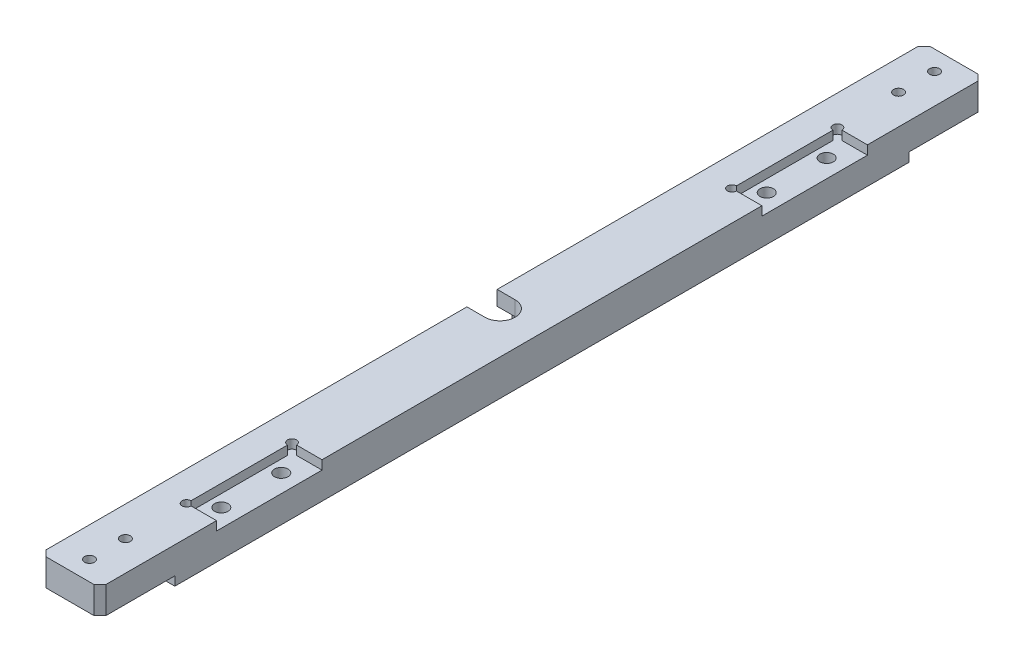
SolidWorks part; units mm, degrees
material "AL6061"
ref_plane "Front Plane" through (0, 0, 0) normal (0, 0, 1) x (1, 0, 0)
ref_plane "Top Plane" through (0, 0, 0) normal (0, 1, 0) x (1, 0, 0)
ref_plane "Right Plane" through (0, 0, 0) normal (1, 0, 0) x (0, 0, -1)
sketch "Sketch1" plane through (0, 0, 0) normal (1, 0, 0) x (0, 0, -1)
  line L1 (-147.5, -6) -> (147.5, -6)
  line L2 (-147.5, -6) -> (-147.5, 6)
  line L3 (-147.5, 6) -> (147.5, 6)
  line L4 (147.5, -6) -> (147.5, 6)
  line L5 (-147.5, -6) -> (147.5, 6) construction
  line L6 (-147.5, 6) -> (147.5, -6) construction
  point P0 (0, 0)
  dimension "D1" = 12
  dimension "D2" = 295
extrude "Boss-Extrude1" add sketch "Sketch1" along normal blind 20
sketch "Sketch2" plane through (0, -6, 0) normal (0, -1, 0) x (1, 0, 0)
  line L0 (0, 0) -> (20, 0) construction
  line L1 (20, 147.5) -> (20, -147.5) construction
  line L2 (0, 0) -> (6, 0) construction
  line L3 (0, 5.05) -> (6, 5.05)
  line L4 (0, -5.05) -> (6, -5.05)
  line L5 (0, 147.5) -> (0, -147.5) construction
  arc A0 (0, 5.05) -> (0, -5.05) centre (0, 0) ccw
  arc A1 (6, -5.05) -> (6, 5.05) centre (6, 0) ccw
  point P5 (3, 0)
  dimension "D2" = 5.05
  dimension "D1" = 3
extrude "Cut-Extrude1" cut sketch "Sketch2" against normal through all
sketch "Sketch3" plane through (0, -6, 0) normal (0, -1, 0) x (1, 0, 0)
  line L0 (0, 0) -> (6, 0) construction
  line L1 (0, 10) -> (6, 10)
  line L2 (0, -10) -> (6, -10)
  arc A0 (0, 10) -> (0, -10) centre (0, 0) ccw
  arc A1 (6, -10) -> (6, 10) centre (6, 0) ccw
  point P4 (3, 0)
  dimension "D1" = 10
extrude "Cut-Extrude2" cut sketch "Sketch3" against normal blind 7.1
sketch "Sketch4" plane through (0, -6, 0) normal (0, 1, 0) x (1, 0, 0)
  line L0 (0, 0) -> (20, 0) construction
  line L1 (20, 147.5) -> (20, -147.5) construction
  line L2 (20, -147.5) -> (20, -122.5)
  line L3 (0, 147.5) -> (20, 147.5)
  line L4 (0, 147.5) -> (0, 122.5)
  line L5 (0, 122.5) -> (20, 122.5)
  line L6 (20, 147.5) -> (20, 122.5)
  line L7 (0, -122.5) -> (20, -122.5)
  line L8 (0, -147.5) -> (0, -122.5)
  line L9 (0, -147.5) -> (20, -147.5)
  dimension "D1" = 25
extrude "Cut-Extrude3" cut sketch "Sketch4" along normal blind 3
sketch "Sketch5" plane through (0, 6, 0) normal (0, 1, 0) x (1, 0, 0)
  line L0 (0, 0) -> (20, 0) construction
  line L1 (20, 147.5) -> (20, -147.5) construction
  line L3 (20, 73.4) -> (10, 73.4)
  line L4 (20, 73.4) -> (20, 108.6)
  line L5 (20, 108.6) -> (10, 108.6)
  line L6 (10, 73.4) -> (10, 108.6)
  line L7 (20, 73.4) -> (10, 108.6) construction
  line L8 (20, 108.6) -> (10, 73.4) construction
  line L9 (20, -108.6) -> (10, -73.4) construction
  line L10 (20, -73.4) -> (10, -108.6) construction
  line L11 (10, -73.4) -> (10, -108.6)
  line L12 (20, -108.6) -> (10, -108.6)
  line L13 (20, -73.4) -> (20, -108.6)
  line L14 (20, -73.4) -> (10, -73.4)
  point P5 (15, 91)
  point P16 (15, -91)
  dimension "D1" = 35.2
  dimension "D2" = 10
  dimension "D3" = 182
extrude "Cut-Extrude4" cut sketch "Sketch5" against normal blind 3
sketch "Sketch7" plane through (0, 6, 0) normal (0, 1, 0) x (1, 0, 0)
  circle A0 centre (10, 108.6) radius 1.5
  circle A1 centre (10, 73.4) radius 1.5
  circle A2 centre (10, -73.4) radius 1.5
  circle A3 centre (10, -108.6) radius 1.5
  dimension "D1" = 3
extrude "Cut-Extrude6" cut sketch "Sketch7" against normal up to surface (3 mm away) up to face at (15, 3, -91)
hole_wizard "M4 Tapped Hole2" positions "Sketch8" profile "Sketch9" tap size "M4" standard "GB"
sketch "Sketch8" plane through (0, -3, 0) normal (0, -1, 0) x (-1, 0, 0)
  point P0 (-10, -141)
  point P3 (-10, -129)
sketch "Sketch9" plane through (10, -3, 141) normal (1, 0, 0) x (0, 0, -1)
  line L0 (0, 0) -> (0, 11.0914)
  line L1 (0, 11.0914) -> (1.65, 10.1)
  line L2 (1.65, 10.1) -> (1.65, 0)
  line L5 (1.65, 0) -> (0, 0)
  line L10 (0, 11.0914) -> (-1.65, 10.1) construction
  line L11 (0, -6.35) -> (0, 107.95) construction
  dimension "螺纹孔钻头直径" = 3.3
  dimension "螺纹孔钻头深度" = 10.1
  dimension "导头角度" = 118
cosmetic thread "Cosmetic Thread1" parameters "D1"=8, "D2"=4
cosmetic thread "Cosmetic Thread2" parameters "D1"=8, "D2"=4
hole_wizard "M4 Tapped Hole1" positions "Sketch10" profile "Sketch11" tap size "M4" standard "GB"
sketch "Sketch10" plane through (0, -3, 0) normal (0, -1, 0) x (-1, 0, 0)
  point P0 (-10, 141)
  point P3 (-10, 129)
sketch "Sketch11" plane through (10, -3, -141) normal (1, 0, 0) x (0, 0, -1)
  line L0 (0, 0) -> (0, 11.0914)
  line L1 (0, 11.0914) -> (1.65, 10.1)
  line L2 (1.65, 10.1) -> (1.65, 0)
  line L5 (1.65, 0) -> (0, 0)
  line L10 (0, 11.0914) -> (-1.65, 10.1) construction
  line L11 (0, -6.35) -> (0, 107.95) construction
  dimension "螺纹孔钻头直径" = 3.3
  dimension "螺纹孔钻头深度" = 10.1
  dimension "导头角度" = 118
cosmetic thread "Cosmetic Thread3" parameters "D1"=8, "D2"=4
cosmetic thread "Cosmetic Thread4" parameters "D1"=8, "D2"=4
hole_wizard "CBORE for M4 Hexagon socket head cap screws1" positions "Sketch12" profile "Sketch13" counterbore size "M4" standard "GB" end condition through all
sketch "Sketch12" plane through (0, -6, 0) normal (0, -1, 0) x (-1, 0, 0)
  point P0 (-14, 101)
  point P3 (-14, 81)
  point P6 (-14, -81)
  point P9 (-14, -101)
sketch "Sketch13" plane through (14, -6, -101) normal (1, 0, 0) x (0, 0, -1)
  line L0 (0, 0) -> (0, 12)
  line L1 (0, 12) -> (2.25, 12)
  line L3 (2.25, 12) -> (2.25, 4.6)
  line L4 (2.25, 4.6) -> (4, 4.6)
  line L5 (4, 4.6) -> (4, 0)
  line L7 (4, 0) -> (0, 0)
  line L11 (0, -6.35) -> (0, 107.95) construction
  dimension "通孔孔直径" = 4.5
  dimension "通孔孔深度" = 12
  dimension "柱形沉头孔直径" = 8
  dimension "柱形沉头孔深度" = 4.6
chamfer "Chamfer1" distance 2 angle 45 4 edges at (0, 1.5, -147.5) (20, 1.5, -147.5) (0, 1.5, 147.5) (20, 1.5, 147.5)
